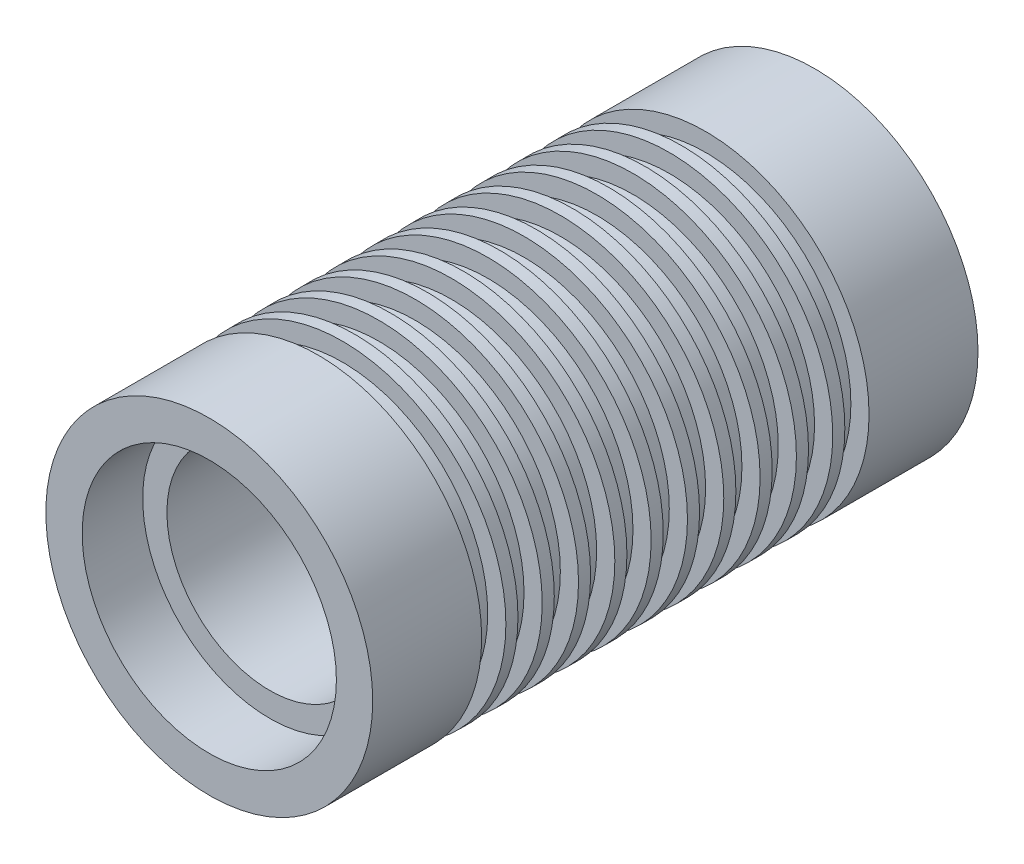
from build123d import *

# Parameters (mm, degrees)
SKETCH_1_R               = 13.5
SKETCH_1_R_2             = 8.5
EXTRUDE_1_DEPTH          = 25
SKETCH_2_W               = 1.5
SKETCH_2_H               = 2
PATTERN_LINEAR_1_COUNT   = 6
PATTERN_LINEAR_1_PITCH   = 3
MIRROR_1_COPY_1_SKETCH_W = 1.5
MIRROR_1_COPY_1_SKETCH_H = 2
MIRROR_1_COPY_2_SKETCH_W = 1.5
MIRROR_1_COPY_2_SKETCH_H = 2
MIRROR_1_COPY_3_SKETCH_W = 1.5
MIRROR_1_COPY_3_SKETCH_H = 2
MIRROR_1_COPY_4_SKETCH_W = 1.5
MIRROR_1_COPY_4_SKETCH_H = 2
MIRROR_1_COPY_5_SKETCH_W = 1.5
MIRROR_1_COPY_5_SKETCH_H = 2
MIRROR_1_COPY_6_SKETCH_W = 1.5
MIRROR_1_COPY_6_SKETCH_H = 2
SKETCH_3_R               = 10.5
CUT_EXTRUDE_1_DEPTH      = 5


with BuildPart() as part:
    # 草图1 → 凸台-拉伸1 (new, symmetric)
    with BuildSketch(Plane.XY):
        Circle(SKETCH_1_R)
        Circle(SKETCH_1_R_2, mode=Mode.SUBTRACT)
    extrude(amount=EXTRUDE_1_DEPTH, both=True)

    # 草图2 → 切除-旋转1 (revolve, cut)
    with BuildSketch(Plane(origin=(0, 0, 0), x_dir=(1, 0, 0), z_dir=(0, 1, 0))):
        with Locations((12.75, 0)):
            Rectangle(SKETCH_2_W, SKETCH_2_H)
    cut_revolve_1 = revolve(axis=Axis((0, 0, 0), (0, 0, -1)), mode=Mode.SUBTRACT)

    # 阵列(线性)1: 切除-旋转1 ×6
    with Locations(*[(0, 0, -i * PATTERN_LINEAR_1_PITCH) for i in range(1, PATTERN_LINEAR_1_COUNT)]):
        add(cut_revolve_1, mode=Mode.SUBTRACT)

    # 镜向1 copy 1 sketch → 镜向1 copy 1 (revolve, cut)
    with BuildSketch(Plane(origin=(0, 0, 3), x_dir=(1, 0, 0), z_dir=(0, 1, 0))):
        with Locations((12.75, 0)):
            Rectangle(MIRROR_1_COPY_1_SKETCH_W, MIRROR_1_COPY_1_SKETCH_H)
    revolve(axis=Axis((0, 0, 3), (0, 0, -1)), mode=Mode.SUBTRACT)

    # 镜向1 copy 2 sketch → 镜向1 copy 2 (revolve, cut)
    with BuildSketch(Plane(origin=(0, 0, 6), x_dir=(1, 0, 0), z_dir=(0, 1, 0))):
        with Locations((12.75, 0)):
            Rectangle(MIRROR_1_COPY_2_SKETCH_W, MIRROR_1_COPY_2_SKETCH_H)
    revolve(axis=Axis((0, 0, 6), (0, 0, -1)), mode=Mode.SUBTRACT)

    # 镜向1 copy 3 sketch → 镜向1 copy 3 (revolve, cut)
    with BuildSketch(Plane(origin=(0, 0, 9), x_dir=(1, 0, 0), z_dir=(0, 1, 0))):
        with Locations((12.75, 0)):
            Rectangle(MIRROR_1_COPY_3_SKETCH_W, MIRROR_1_COPY_3_SKETCH_H)
    revolve(axis=Axis((0, 0, 9), (0, 0, -1)), mode=Mode.SUBTRACT)

    # 镜向1 copy 4 sketch → 镜向1 copy 4 (revolve, cut)
    with BuildSketch(Plane(origin=(0, 0, 12), x_dir=(1, 0, 0), z_dir=(0, 1, 0))):
        with Locations((12.75, 0)):
            Rectangle(MIRROR_1_COPY_4_SKETCH_W, MIRROR_1_COPY_4_SKETCH_H)
    revolve(axis=Axis((0, 0, 12), (0, 0, -1)), mode=Mode.SUBTRACT)

    # 镜向1 copy 5 sketch → 镜向1 copy 5 (revolve, cut)
    with BuildSketch(Plane(origin=(0, 0, 15), x_dir=(1, 0, 0), z_dir=(0, 1, 0))):
        with Locations((12.75, 0)):
            Rectangle(MIRROR_1_COPY_5_SKETCH_W, MIRROR_1_COPY_5_SKETCH_H)
    revolve(axis=Axis((0, 0, 15), (0, 0, -1)), mode=Mode.SUBTRACT)

    # 镜向1 copy 6 sketch → 镜向1 copy 6 (revolve, cut)
    with BuildSketch(Plane(origin=(0, 0, 0), x_dir=(1, 0, 0), z_dir=(0, 1, 0))):
        with Locations((12.75, 0)):
            Rectangle(MIRROR_1_COPY_6_SKETCH_W, MIRROR_1_COPY_6_SKETCH_H)
    revolve(axis=Axis((0, 0, 0), (0, 0, -1)), mode=Mode.SUBTRACT)

    # 草图3 → 切除-拉伸1 (cut)
    with BuildSketch(Plane.XY.offset(25)):
        Circle(SKETCH_3_R)
    cut_extrude_1 = extrude(amount=-CUT_EXTRUDE_1_DEPTH, mode=Mode.SUBTRACT)

    # 镜向2: 切除-拉伸1 across plane
    add(cut_extrude_1.mirror(Plane.XY), mode=Mode.SUBTRACT)


solid = part.part
